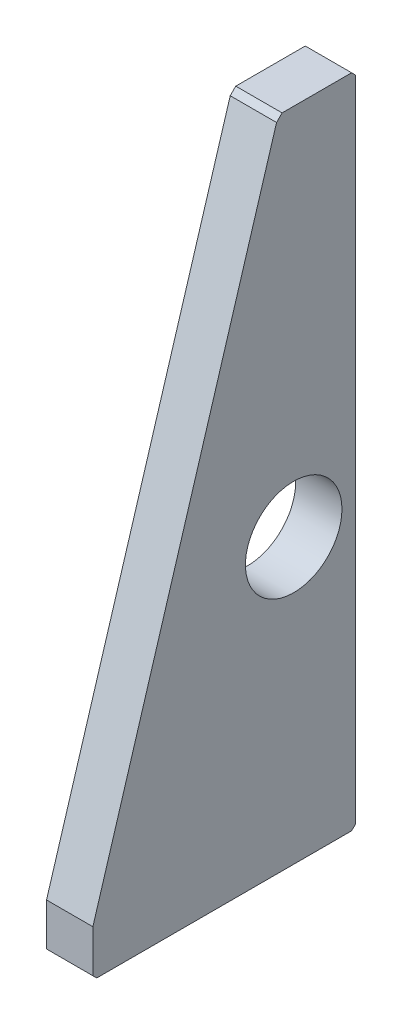
from build123d import *
from OCP.BRepFilletAPI import BRepFilletAPI_MakeChamfer

# Parameters (mm, degrees)
BOSS_EXTRUDE1_DEPTH   = 6
M5_TAPPED_HOLE1_D     = 4.2
M5_TAPPED_HOLE1_DEPTH = 12.4
M5_TAPPED_HOLE1_TIP   = 1.2618073
M5_TAPPED_HOLE2_D     = 4.2
M5_TAPPED_HOLE2_DEPTH = 12.4
M5_TAPPED_HOLE2_TIP   = 1.2618073
CHAMFER1_SIZE         = 1
CHAMFER1_SIZE2        = 1.501184106
SKETCH6_R             = 12.5
CUT_EXTRUDE1_DEPTH    = 184.488419253


with BuildPart() as part:
    # Sketch1 → Boss-Extrude1 (new, symmetric)
    with BuildSketch(Plane(origin=(0, 0, 0), x_dir=(0, 0, -1), z_dir=(1, 0, 0))):
        Polygon((0, 0), (-68, 0), (-68, 12), (-20, 170), (0, 170), align=None)
    extrude(amount=BOSS_EXTRUDE1_DEPTH, both=True)

    # M5 Tapped Hole1
    with Locations(Plane(origin=(0, 0, 0), x_dir=(-1, 0, 0), z_dir=(0, 0, -1))):
        with Locations((0, 20), (0, 155)):
            Hole(M5_TAPPED_HOLE1_D / 2, depth=M5_TAPPED_HOLE1_DEPTH)
            with Locations((0, 0, -(M5_TAPPED_HOLE1_DEPTH + M5_TAPPED_HOLE1_TIP / 2))):  # 118° drill point
                Cone(0, M5_TAPPED_HOLE1_D / 2, M5_TAPPED_HOLE1_TIP, mode=Mode.SUBTRACT)

    # M5 Tapped Hole2
    with Locations(Plane(origin=(0, 0, 0), x_dir=(-1, 0, 0), z_dir=(0, -1, 0))):
        with Locations((0, -58), (0, -10)):
            Hole(M5_TAPPED_HOLE2_D / 2, depth=M5_TAPPED_HOLE2_DEPTH)
            with Locations((0, 0, -(M5_TAPPED_HOLE2_DEPTH + M5_TAPPED_HOLE2_TIP / 2))):  # 118° drill point
                Cone(0, M5_TAPPED_HOLE2_D / 2, M5_TAPPED_HOLE2_TIP, mode=Mode.SUBTRACT)

    # Chamfer1: one chamfer whose edges measure the first distance from different faces: ONE call of the kernel's chamfer builder (chamfer() names one face for all edges)
    chamfer1_edges_1 = [part.edges().sort_by_distance(p)[0] for p in [
        (0, 0, 0),
        (0, 0, 68),
        (0, 170, 0),
    ]]
    chamfer1_edges_2 = [part.edges().sort_by_distance(p)[0] for p in [
        (0, 170, 20),
    ]]
    chamfer1_side_2 = [part.faces().sort_by_distance(p)[0] for p in [
        (0, 170, 10),
    ]]
    chamfer1 = BRepFilletAPI_MakeChamfer(part.part.solid().wrapped)
    for e in chamfer1_edges_1:
        chamfer1.Add(CHAMFER1_SIZE, e.wrapped)
    for e in chamfer1_edges_2:
        chamfer1.Add(CHAMFER1_SIZE, CHAMFER1_SIZE2, e.wrapped, chamfer1_side_2[0].wrapped)  # the first distance lies on this face
    add(Compound.cast(chamfer1.Shape()), mode=Mode.REPLACE)

    # Sketch6 → Cut-Extrude1 (cut, through all)
    with BuildSketch(Plane(origin=(6, 0, 0), x_dir=(0, 0, -1), z_dir=(1, 0, 0))):
        with Locations((-16, 73.4)):
            Circle(SKETCH6_R)
    extrude(amount=-CUT_EXTRUDE1_DEPTH, mode=Mode.SUBTRACT)


solid = part.part
